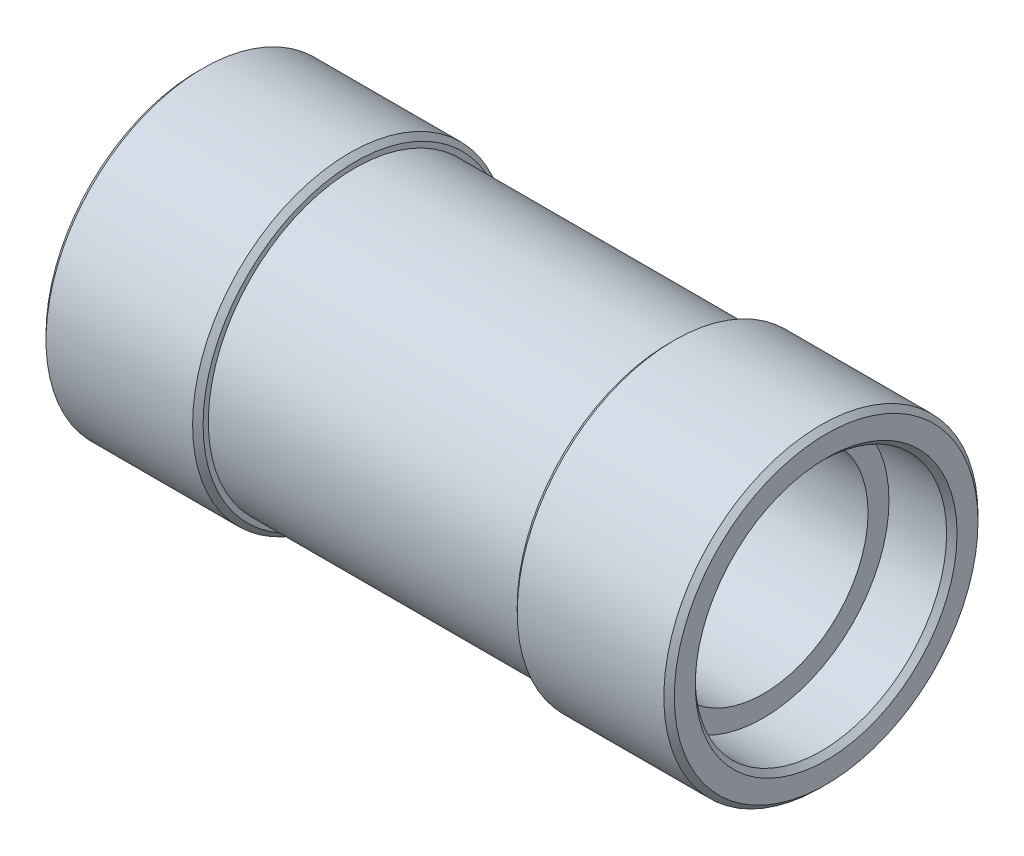
SolidWorks part; units mm, degrees
material "SUS304"
ref_plane "Front Plane" through (0, 0, 0) normal (0, 0, 1) x (1, 0, 0)
ref_plane "Top Plane" through (0, 0, 0) normal (0, 1, 0) x (1, 0, 0)
ref_plane "Right Plane" through (0, 0, 0) normal (1, 0, 0) x (0, 0, -1)
sketch "Sketch1" plane through (0, 0, 0) normal (0, 0, 1) x (1, 0, 0)
  line L0 (48.5337, 0) -> (-48.5337, 0) construction
  line L1 (-24, 10) -> (-24, 12)
  line L2 (-24, 12) -> (-30, 12)
  line L3 (-30, 12) -> (-30, 15)
  line L4 (-30, 15) -> (30, 15)
  line L5 (-24, 10) -> (24, 10)
  line L6 (0, 0) -> (0, 15) construction
  line L7 (30, 12) -> (30, 15)
  line L8 (24, 12) -> (30, 12)
  line L9 (24, 10) -> (24, 12)
  line L11 (-15, 16) -> (15, 16)
  line L12 (-15, 16) -> (-15, 14)
  line L13 (-15, 14) -> (15, 14)
  line L14 (15, 16) -> (15, 14)
  line L15 (-15, 16) -> (15, 14) construction
  line L16 (-15, 14) -> (15, 16) construction
  point P12 (0, 10)
  dimension "D1" = 30
  dimension "D2" = 24
  dimension "D3" = 20
  dimension "D4" = 6
  dimension "D5" = 60
  dimension "D6" = 30
  dimension "D7" = 1
revolve "Revolve1" add sketch "Sketch1" angle 360 about L0
chamfer "Chamfer1" distance 0.5 angle 45 6 edges at (30, 0, -12) (30, 0, -15) (-30, 0, -12) (-30, 0, -15) (15, 0, -15) (-15, 0, -15)
